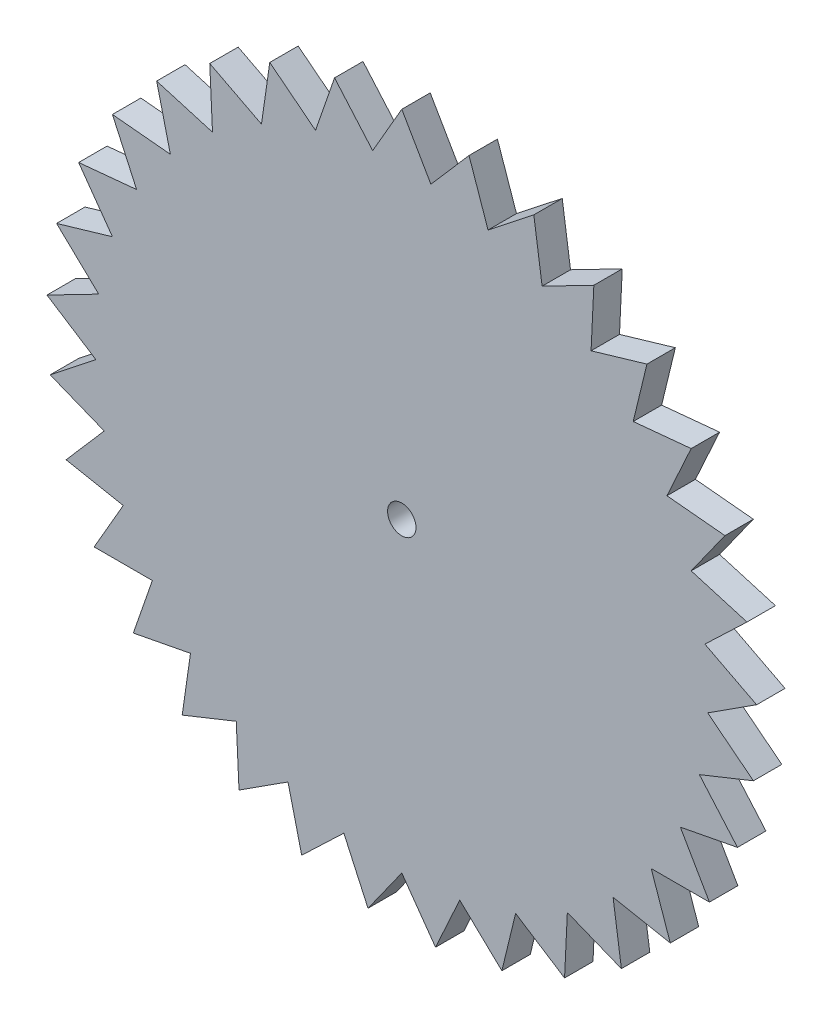
SolidWorks part; units mm, degrees
ref_plane "前视基准面" through (0, 0, 0) normal (0, 0, 1) x (1, 0, 0)
ref_plane "上视基准面" through (0, 0, 0) normal (0, 1, 0) x (1, 0, 0)
ref_plane "右视基准面" through (0, 0, 0) normal (1, 0, 0) x (0, 0, -1)
other "Configuration Table"
sketch "草图1" plane through (0, 0, 0) normal (0, 0, 1) x (1, 0, 0)
  line L0 (0, 0) -> (0, 142.3372) construction
  line L1 (0, 125) -> (-10.2421, 107.2602)
  line L2 (0, 125) -> (10.2421, 107.2602)
  line L3 (23.6564, 122.7411) -> (10.2421, 107.2602)
  line L4 (23.6564, 122.7411) -> (30.3561, 103.3835)
  line L5 (46.4578, 116.046) -> (30.3561, 103.3835)
  line L6 (46.4578, 116.046) -> (49.373, 95.7703)
  line L7 (67.5801, 105.1567) -> (49.373, 95.7703)
  line L8 (67.5801, 105.1567) -> (66.6054, 84.6957)
  line L9 (86.2599, 90.4668) -> (66.6054, 84.6957)
  line L10 (86.2599, 90.4668) -> (81.4305, 70.56)
  line L11 (101.822, 72.5071) -> (81.4305, 70.56)
  line L12 (101.822, 72.5071) -> (93.3125, 53.874)
  line L13 (113.704, 51.9269) -> (93.3125, 53.874)
  line L14 (113.704, 51.9269) -> (101.822, 35.2409)
  line L15 (121.4764, 29.4699) -> (101.822, 35.2409)
  line L16 (121.4764, 29.4699) -> (106.6513, 15.3341)
  line L17 (124.8584, 5.9477) -> (106.6513, 15.3341)
  line L18 (124.8584, 5.9477) -> (107.626, -5.1269)
  line L19 (123.7277, -17.7894) -> (107.626, -5.1269)
  line L20 (123.7277, -17.7894) -> (104.7108, -25.4026)
  line L21 (118.1251, -40.8835) -> (104.7108, -25.4026)
  line L22 (118.1251, -40.8835) -> (98.0111, -44.7602)
  line L23 (108.2532, -62.5) -> (98.0111, -44.7602)
  line L24 (108.2532, -62.5) -> (87.769, -62.5)
  line L25 (94.4687, -81.8576) -> (87.769, -62.5)
  line L26 (94.4687, -81.8576) -> (74.3547, -77.9809)
  line L27 (77.2699, -98.2566) -> (74.3547, -77.9809)
  line L28 (77.2699, -98.2566) -> (58.253, -90.6434)
  line L29 (57.2783, -111.1044) -> (58.253, -90.6434)
  line L30 (57.2783, -111.1044) -> (40.0459, -100.0298)
  line L31 (35.2166, -119.9366) -> (40.0459, -100.0298)
  line L32 (35.2166, -119.9366) -> (20.3915, -105.8009)
  line L33 (11.882, -124.434) -> (20.3915, -105.8009)
  line L34 (11.882, -124.434) -> (0, -107.748)
  line L35 (-11.882, -124.434) -> (0, -107.748)
  line L36 (-11.882, -124.434) -> (-20.3915, -105.8009)
  line L37 (-35.2166, -119.9366) -> (-20.3915, -105.8009)
  line L38 (-35.2166, -119.9366) -> (-40.0459, -100.0298)
  line L39 (-57.2783, -111.1044) -> (-40.0459, -100.0298)
  line L40 (-57.2783, -111.1044) -> (-58.253, -90.6434)
  line L41 (-77.2699, -98.2566) -> (-58.253, -90.6434)
  line L42 (-77.2699, -98.2566) -> (-74.3547, -77.9809)
  line L43 (-94.4687, -81.8576) -> (-74.3547, -77.9809)
  line L44 (-94.4687, -81.8576) -> (-87.769, -62.5)
  line L45 (-108.2532, -62.5) -> (-87.769, -62.5)
  line L46 (-108.2532, -62.5) -> (-98.0111, -44.7602)
  line L47 (-118.1251, -40.8835) -> (-98.0111, -44.7602)
  line L48 (-118.1251, -40.8835) -> (-104.7108, -25.4026)
  line L49 (-123.7277, -17.7894) -> (-104.7108, -25.4026)
  line L50 (-123.7277, -17.7894) -> (-107.626, -5.1269)
  line L51 (-124.8584, 5.9477) -> (-107.626, -5.1269)
  line L52 (-124.8584, 5.9477) -> (-106.6513, 15.3341)
  line L53 (-121.4764, 29.4699) -> (-106.6513, 15.3341)
  line L54 (-121.4764, 29.4699) -> (-101.822, 35.2409)
  line L55 (-113.704, 51.9269) -> (-101.822, 35.2409)
  line L56 (-113.704, 51.9269) -> (-93.3125, 53.874)
  line L57 (-101.822, 72.5071) -> (-93.3125, 53.874)
  line L58 (-101.822, 72.5071) -> (-81.4305, 70.56)
  line L59 (-86.2599, 90.4668) -> (-81.4305, 70.56)
  line L60 (-86.2599, 90.4668) -> (-66.6054, 84.6957)
  line L61 (-67.5801, 105.1567) -> (-66.6054, 84.6957)
  line L62 (-67.5801, 105.1567) -> (-49.373, 95.7703)
  line L63 (-46.4578, 116.046) -> (-49.373, 95.7703)
  line L64 (-46.4578, 116.046) -> (-30.3561, 103.3835)
  line L65 (-23.6564, 122.7411) -> (-30.3561, 103.3835)
  line L66 (-23.6564, 122.7411) -> (-10.2421, 107.2602)
  line L67 (0, 0) -> (10.6293, 106.5894) construction
  circle A0 centre (0, 0) radius 125 construction
  circle A3 centre (0, 0) radius 5
  dimension "D1" = 250
  dimension "D2" = 60
  dimension "D4" = 107.1181
  dimension "D3" = 33
extrude "凸台-拉伸4" add sketch "草图1" along normal blind 10
